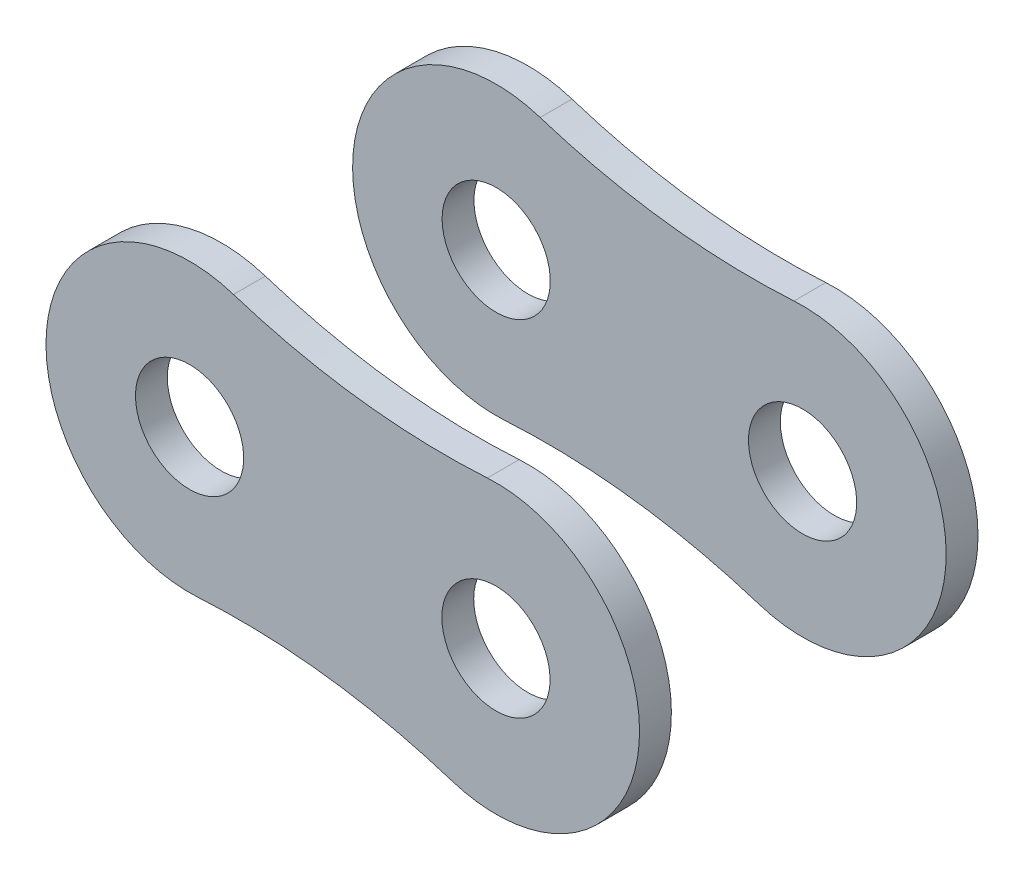
from build123d import *

# Parameters (mm, degrees)
SKETCH_2_R        = 4.255
EXTRUDE_1_DEPTH   = 3.875
EXTRUDE_1_2_DEPTH = 3.875
EXTRUDE_2_DEPTH   = 1.775
SKETCH_6_R        = 2.225
EXTRUDE_4_DEPTH   = 1.31


with BuildPart() as part:
    # 草图2 → 拉伸1 (new, symmetric)
    with BuildSketch(Plane.XY):
        with Locations((6.35, 0)):
            Circle(SKETCH_2_R)
    extrude(amount=EXTRUDE_1_DEPTH, both=True)



with BuildPart() as body_2:
    # 草图2 → Extrude 1 2 (new, symmetric)
    with BuildSketch(Plane.XY):
        with Locations((-6.35, 0)):
            Circle(SKETCH_2_R)
    extrude(amount=EXTRUDE_1_2_DEPTH, both=True)


with BuildPart() as part_1:
    add(part.part)

    add(body_2.part)  # 拉伸2 merges body 2
    # 草图3 → 拉伸2 (add)
    with BuildSketch(Plane.XY.offset(3.875)):
        with BuildLine():
            ThreePointArc((-5.261178614, 5.803748184), (-12.255, 0), (-5.261178614, -5.803748184))
            ThreePointArc((-5.261178614, -5.803748184), (0, -5.3145), (5.261178614, -5.803748184))
            ThreePointArc((5.261178614, -5.803748184), (12.255, 0), (5.261178614, 5.803748184))
            ThreePointArc((5.261178614, 5.803748184), (0, 5.3145), (-5.261178614, 5.803748184))
        make_face()
    extrude(amount=EXTRUDE_2_DEPTH)


with BuildPart() as body_2_2:
    # 草图6 → 拉伸4 (new body)
    with BuildSketch(Plane.XY.offset(5.65)):
        with BuildLine():
            ThreePointArc((17.144009153, -7.210570587), (24.808872428, -2.327241646), (18.595954811, 4.305758071))
            ThreePointArc((18.595954811, 4.305758071), (13.314900062, 4.478457031), (8.156242384, 5.621967045))
            ThreePointArc((8.156242384, 5.621967045), (0.491379108, 0.738638104), (6.704296726, -5.894361613))
            ThreePointArc((6.704296726, -5.894361613), (11.985351475, -6.067060574), (17.144009153, -7.210570587))
        make_face()
        with Locations(Location((6.35, 0, 0), (0, 0, 180))):
            Circle(SKETCH_6_R, mode=Mode.SUBTRACT)
        with Locations(Location((18.950251537, -1.588603542, 0), (0, 0, 180))):
            Circle(SKETCH_6_R, mode=Mode.SUBTRACT)
    extrude(amount=EXTRUDE_4_DEPTH)


with BuildPart() as body_2_3:
    # 镜向1: mirrored copy
    add(body_2_2.part.mirror(Plane(origin=(0, 0, 0), x_dir=(1, 0, 0), z_dir=(0, 0, -1))))


solid = Compound([body_2_2.part, body_2_3.part])
